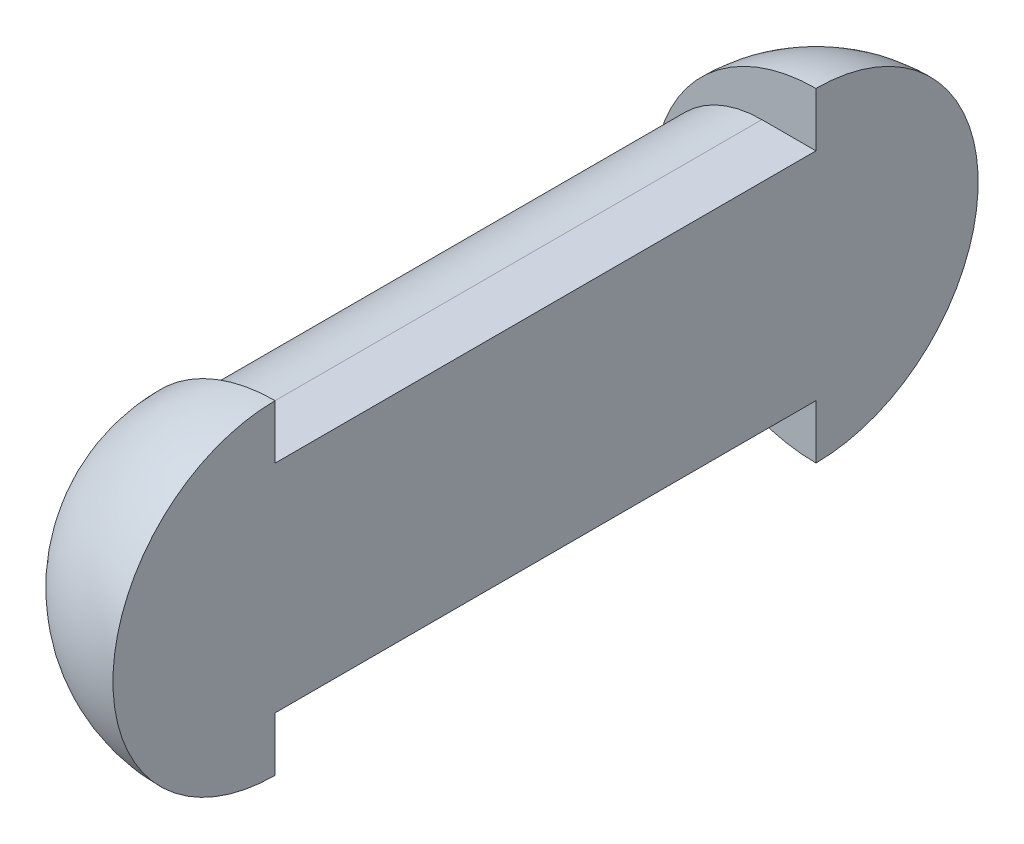
from build123d import *

# Parameters (mm, degrees)
EXTRUDE_1_DEPTH = 100
REVOLVE_1_ANGLE = 90


with BuildPart() as part:
    # 草图1 → 凸台-拉伸1 (new body)
    with BuildSketch(Plane.XY):
        with BuildLine():
            Line((0, 0), (0, -80))
            Line((0, -80), (-20, -80))
            ThreePointArc((-20, -80), (-60, -40), (-20, 0))
            Line((-20, 0), (0, 0))
        make_face()
    extrude_1 = extrude(amount=-EXTRUDE_1_DEPTH)

    # 草图2 → 旋转1 (revolve)
    with BuildSketch(Plane(origin=(0, 0, 0), x_dir=(0, 0, -1), z_dir=(1, 0, 0))):
        with BuildLine():
            Line((100, 20), (100, -100))
            ThreePointArc((100, -100), (160, -40), (100, 20))
        make_face()
    revolve_1 = revolve(axis=Axis((0, 20, -100), (0, 1, 0)), revolution_arc=REVOLVE_1_ANGLE)

    # 镜向1: 凸台-拉伸1, 旋转1 across plane
    add(extrude_1.mirror(Plane(origin=(-20, -40, 0), x_dir=(1, 0, 0), z_dir=(0, 0, -1))))
    add(revolve_1.mirror(Plane(origin=(-20, -40, 0), x_dir=(1, 0, 0), z_dir=(0, 0, -1))))


solid = part.part
